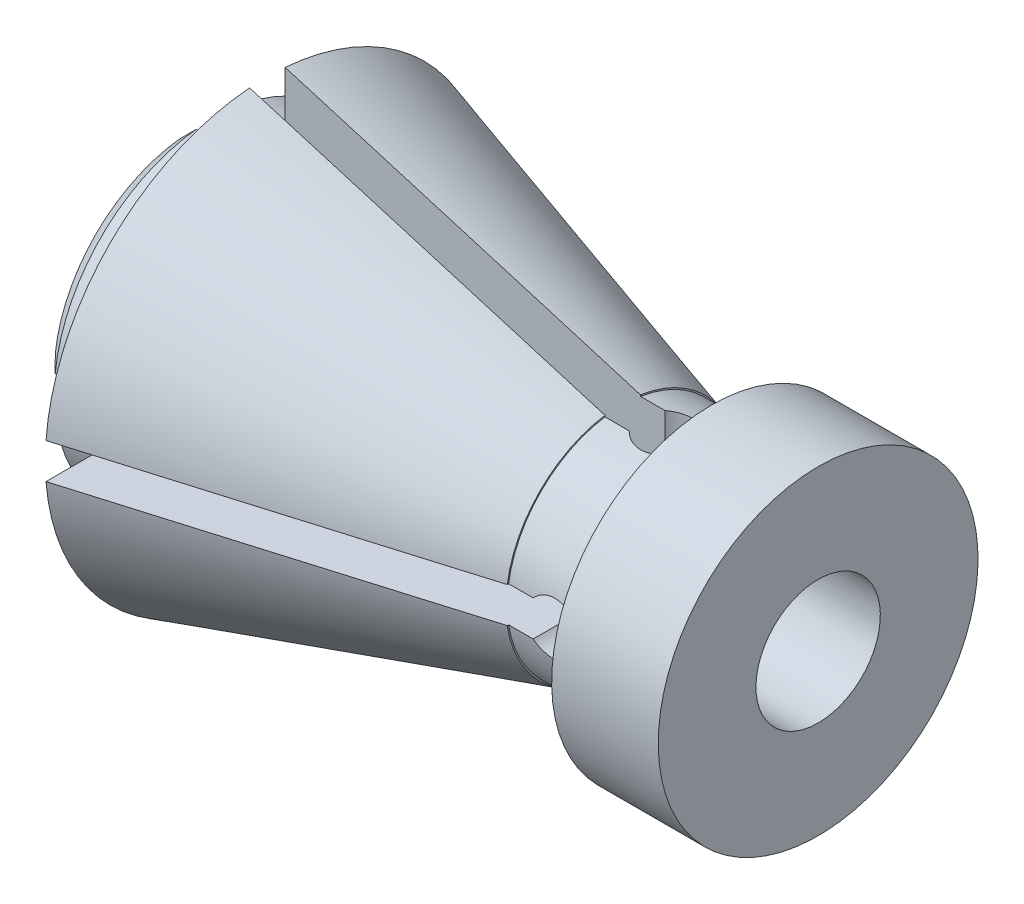
from build123d import *

# Parameters (mm, degrees)
SKETCH2_R               = 3.5
CUT_EXTRUDE1_DEPTH      = 40.210967853
CUT_EXTRUDE2_DEPTH      = 40.210967853
CUT_EXTRUDE2_DEPTH_BACK = 40.210967853
SKETCH3_R               = 1.5
CUT_EXTRUDE3_DEPTH      = 40.210967943
CUT_EXTRUDE3_DEPTH_BACK = 40.210967943
SKETCH4_R               = 1.5
CUT_EXTRUDE4_DEPTH      = 40.210967943
CUT_EXTRUDE4_DEPTH_BACK = 40.210967943
SKETCH5_W               = 50.763932022
SKETCH5_H               = 2
CUT_EXTRUDE5_DEPTH      = 40.198214334
CUT_EXTRUDE5_DEPTH_BACK = 40.198214334
SKETCH6_W               = 50.763932022
SKETCH6_H               = 2
CHAMFER1_SIZE           = 1


with BuildPart() as part:
    # Sketch1 → Revolve1 (revolve)
    with BuildSketch(Plane.XY):
        Polygon((0, 0), (0, 9), (4, 9), (4, 12.5), (24, 6.575730101), (24, 6.5), (29, 6.5), (29, 9), (35, 9), (35, 0), align=None)
    revolve(axis=Axis((35, 0, 0), (-1, 0, 0)))

    # Sketch2 → Cut-Extrude1 (cut, through all)
    with BuildSketch(Plane.ZY):
        with Locations(Location((0, 0, 0), (0, 0, 270))):
            Circle(SKETCH2_R)
    extrude(amount=-CUT_EXTRUDE1_DEPTH, mode=Mode.SUBTRACT)

    # Sketch3 → Cut-Extrude2 (cut, two sides: drawn at the far end of the back side and taken through both)
    with BuildSketch(Plane.XY.offset(-CUT_EXTRUDE2_DEPTH_BACK)):
        with Locations((26.5, 0)):
            Circle(SKETCH3_R)
    extrude(amount=CUT_EXTRUDE2_DEPTH + CUT_EXTRUDE2_DEPTH_BACK, mode=Mode.SUBTRACT)

    # Sketch4 → Cut-Extrude3 (cut, two sides: drawn at the far end of the back side and taken through both)
    with BuildSketch(Plane(origin=(0, 0, 0), x_dir=(1, 0, 0), z_dir=(0, 1, 0)).offset(-CUT_EXTRUDE3_DEPTH_BACK)):
        with Locations(Location((26.5, 0, 0), (0, 0, 270))):
            Circle(SKETCH4_R)
    extrude(amount=CUT_EXTRUDE3_DEPTH + CUT_EXTRUDE3_DEPTH_BACK, mode=Mode.SUBTRACT)

    # Sketch5 → Cut-Extrude4 (cut, two sides: drawn at the far end of the back side and taken through both)
    with BuildSketch(Plane.XY.offset(-CUT_EXTRUDE4_DEPTH_BACK)):
        Rectangle(SKETCH5_W, SKETCH5_H)
    extrude(amount=CUT_EXTRUDE4_DEPTH + CUT_EXTRUDE4_DEPTH_BACK, mode=Mode.SUBTRACT)

    # Sketch6 → Cut-Extrude5 (cut, two sides: drawn at the far end of the back side and taken through both)
    with BuildSketch(Plane(origin=(0, 0, 0), x_dir=(1, 0, 0), z_dir=(0, 1, 0)).offset(-CUT_EXTRUDE5_DEPTH_BACK)):
        Rectangle(SKETCH6_W, SKETCH6_H)
    extrude(amount=CUT_EXTRUDE5_DEPTH + CUT_EXTRUDE5_DEPTH_BACK, mode=Mode.SUBTRACT)

    # Chamfer1
    chamfer1_edges = [part.edges().sort_by_distance(p)[0] for p in [
        (0, 6.363961031, 6.363961031),
        (0, -6.363961031, -6.363961031),
        (0, -6.363961031, 6.363961031),
        (0, 6.363961031, -6.363961031),
    ]]
    chamfer(chamfer1_edges, length=CHAMFER1_SIZE)


solid = part.part
